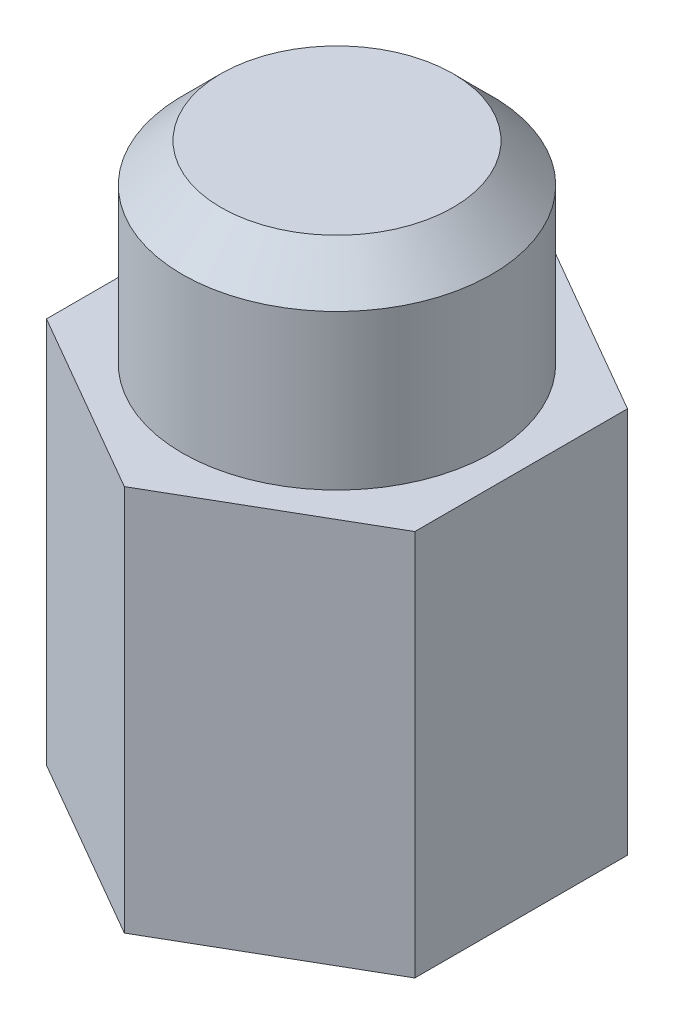
SolidWorks part; units mm, degrees
ref_plane "Front Plane" through (0, 0, 0) normal (0, 0, 1) x (1, 0, 0)
ref_plane "Top Plane" through (0, 0, 0) normal (0, 1, 0) x (1, 0, 0)
ref_plane "Right Plane" through (0, 0, 0) normal (1, 0, 0) x (0, 0, -1)
sketch "Sketch1" plane through (0, 0, 0) normal (0, 1, 0) x (1, 0, 0)
  line L1 (0, 5.5) -> (-4.7631, 2.75)
  line L2 (-4.7631, 2.75) -> (-4.7631, -2.75)
  line L3 (-4.7631, -2.75) -> (0, -5.5)
  line L4 (0, -5.5) -> (4.7631, -2.75)
  line L5 (4.7631, -2.75) -> (4.7631, 2.75)
  line L6 (4.7631, 2.75) -> (0, 5.5)
  circle A0 centre (0, 0) radius 4.7631 construction
  dimension "D1" = 11
extrude "Boss-Extrude1" add sketch "Sketch1" along normal mid plane 10
sketch "Sketch3" plane through (0, 5, 0) normal (0, 1, 0) x (1, 0, 0)
  circle A0 centre (0, 0) radius 4
  dimension "D1" = 8
extrude "Boss-Extrude2" add sketch "Sketch3" along normal blind 5
chamfer "Chamfer1" distance 1 angle 45 1 edges at (0, 10, 4)
hole_wizard "M6x1.0 Tapped Hole1" positions "Sketch5" profile "Sketch4" tap size "M6x1.0" standard "ANSI Metric"
sketch "Sketch5" plane through (0, -5, 0) normal (0, -1, 0) x (-1, 0, 0)
  point P0 (-0.0014, 0)
sketch "Sketch4" plane through (0.0014, -5, 0) normal (1, 0, 0) x (0, 0, -1)
  line L0 (0, 0) -> (0, 9.5022)
  line L1 (0, 9.5022) -> (2.5, 8)
  line L2 (2.5, 8) -> (2.5, 0)
  line L5 (2.5, 0) -> (0, 0)
  line L10 (0, 9.5022) -> (-2.5, 8) construction
  line L11 (0, -6.35) -> (0, 107.95) construction
  dimension "Tap Drill Dia." = 5
  dimension "Tap Drill Depth" = 8
  dimension "Drill Angle" = 118
cosmetic thread "Hole Thread1" parameters "D1"=4, "D2"=6
